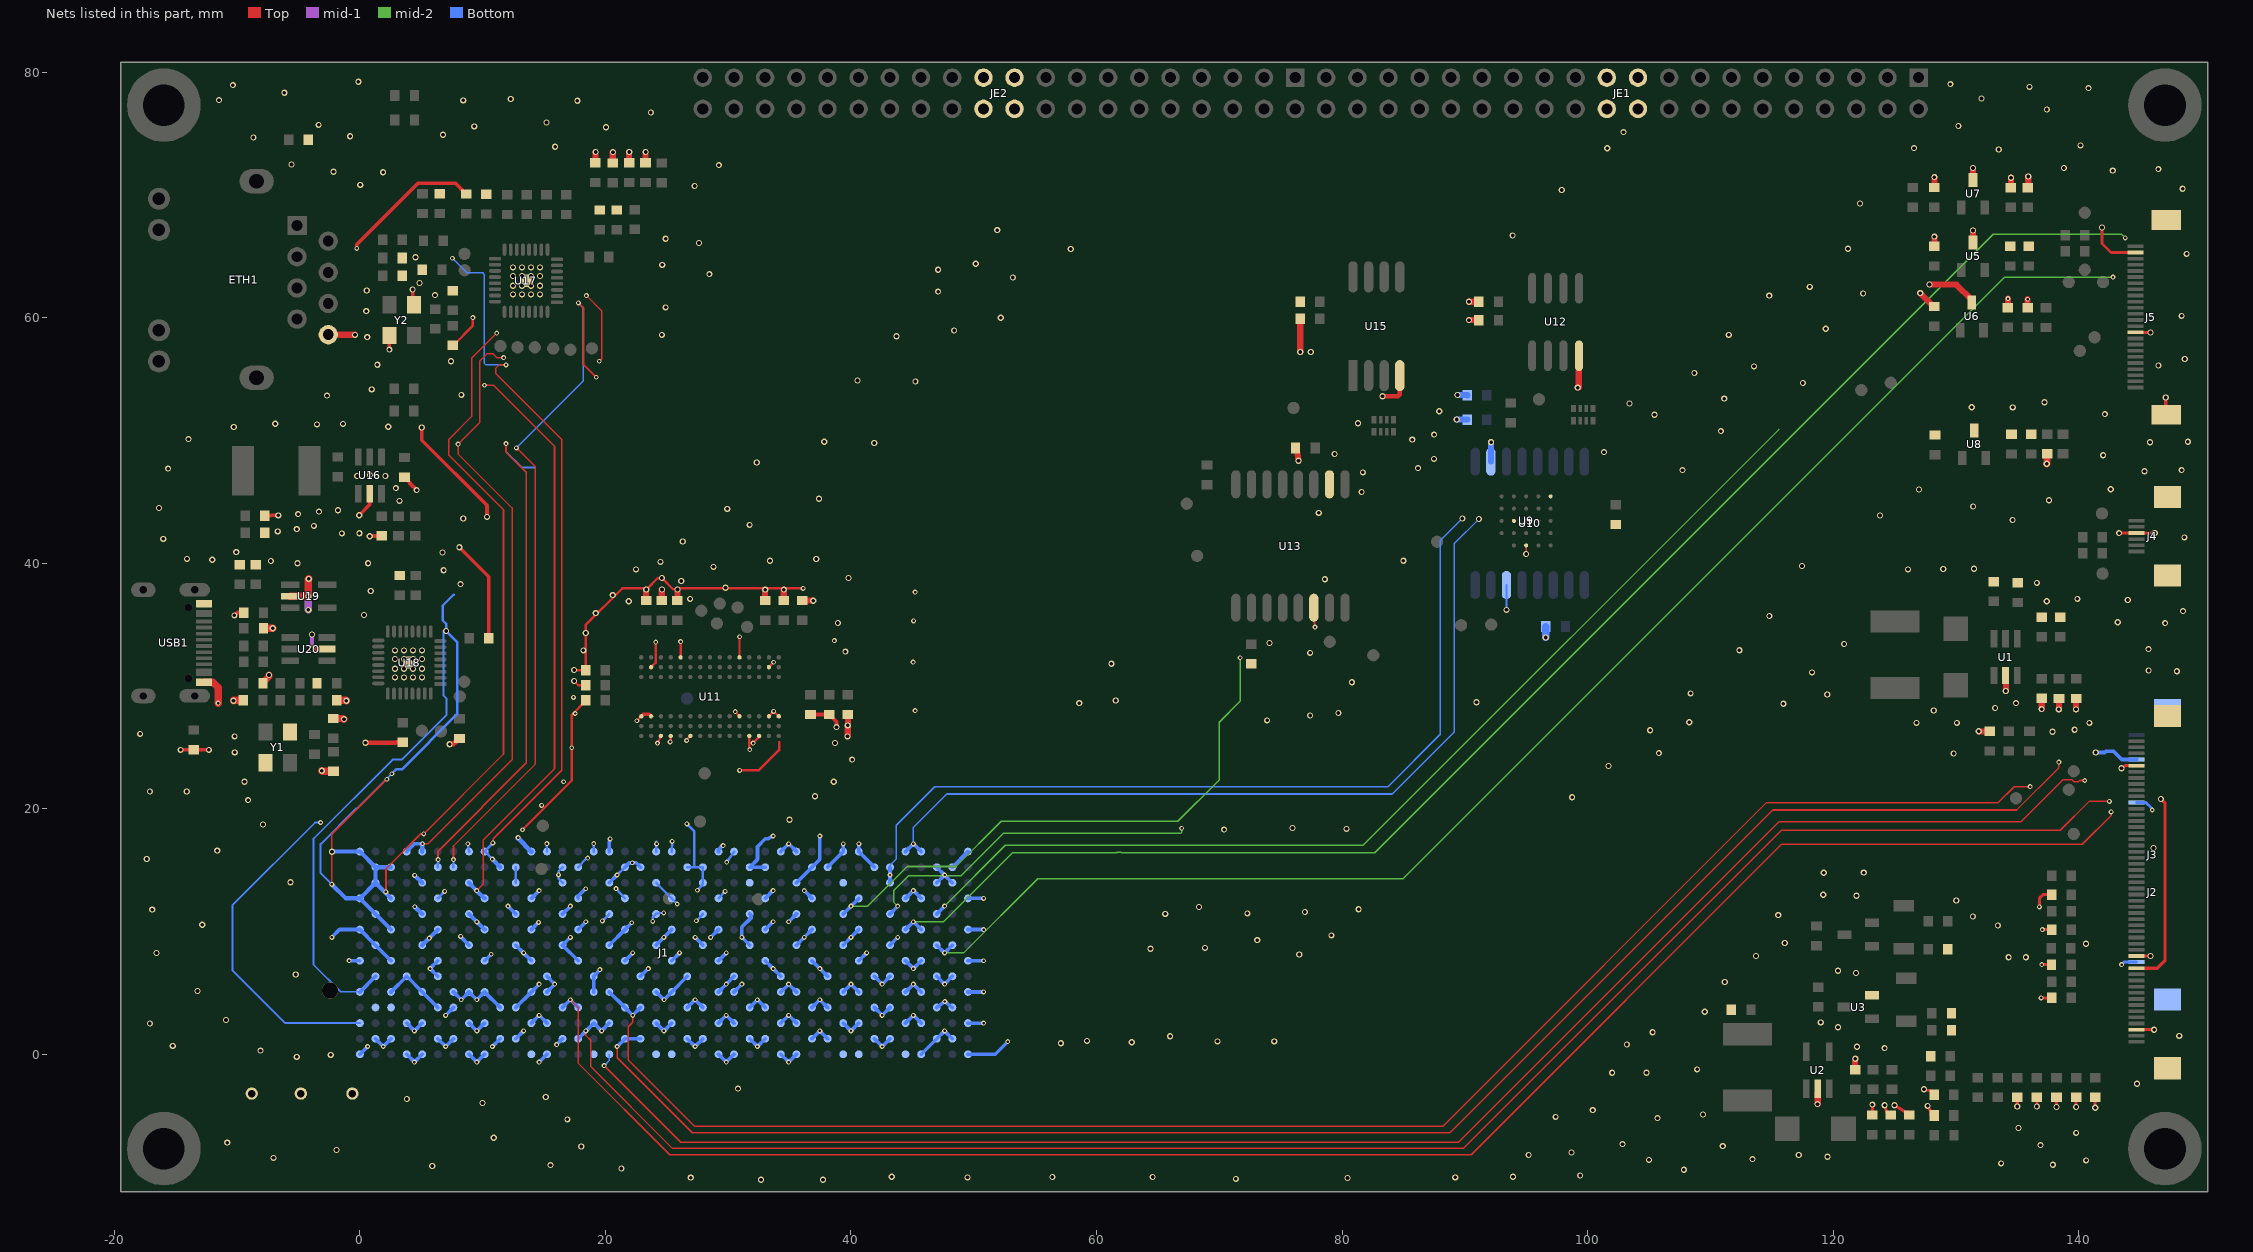
[diagram p0: the nets of this part, all layers, seen from the top]
# Altium PCB MISC105414.PcbDoc (part 6 of 11)
Units mm, origin at the board's own origin, x right, y up, seen from the top; angles counter-clockwise.
Board outline 170 x 92 mm, 6 copper layers (Top, GND, mid-1, mid-2, mid-3, Bottom), stack 1.231 mm thick; 238 components, 304 nets, 1456 pads, 1258 vias.
Unrouted connection lines stored in the file: 57.

## Via types
v1: diameter 0.4, hole 0.2, Top to Bottom, tented top, 618 vias
v2: diameter 0.5, hole 0.3, Top to Bottom, tented top, 522 vias
v3: diameter 0.5, hole 0.3, Top to Bottom, 41 vias
v4: diameter 1, hole 0.5, Top to Bottom, tented top, 36 vias
v5: diameter 0.7, hole 0.4, Top to Bottom, tented top, 34 vias
v6: diameter 1.3, hole 1.3, Top to Bottom, tented top, 3 vias
v7: diameter 4, hole 4, Top to Bottom, tented top, 2 vias
v8: diameter 3.3, hole 3.3, Top to Bottom, tented top, 2 vias

## Nets (pads, with @x,y where several pads share a name; then routed paths per layer and width w, separated by ;. In a path a pad name is that pad's centre, name@x,y a point inside that pad or via, vN(x,y) a via of type N, cw(c..) or ccw(c..) an arc to the next point about the centre after c; other vN are vias at no path point) (continued)
GND: C1.2 C3.2 C4.2 C5.1 C6.1 C7.1 C8.1 C9.2 C10.2 C11.2 C15.2 C17.2 C18.2 C19.1 C20.2 C21.2 C22.2 C27.2 C28.2 C29.2 C30.2 C31.2 C32.2 C33.2 C34.2 C35.1 C36.1 C37.1 C38.1 C39.2 C40.2 C41.2 C42.1 C43.1 C44.1 C45.2 C46.1 C47.1 C48.1 C49.1 C50.1 C51.1 C52.1 C53.1 C54.1 C55.1 C56.1 C65.2 C66.2 C67.1 C68.1 C69.2 C70.2 C71.2 C72.2 C73.1 C74.1 C75.1 C77.1 C78.1 C79.1 C80.2 C82.2 C83.2 C84.2 C85.2 C86.2 C87.1 C88.2 C89.1 C90.1 C91.1 C92.2 C93.2 C94.1 C95.1 ETH1.8 J1.A1 J1.A4 J1.A5 J1.A8 J1.A9 J1.A12 J1.A13 J1.A16 J1.A17 J1.A20 J1.A21 J1.A24 J1.A25 J1.A28 J1.A29 J1.A32 J1.A33 J1.A36 J1.A37 J1.A40 J1.B2 J1.B3 J1.B6 J1.B7 J1.B10 J1.B11 J1.B14 J1.B15 J1.B18 J1.B19 J1.B22 J1.B23 J1.B26 J1.B27 J1.B30 J1.B31 J1.B34 J1.B35 J1.B38 J1.B39 J1.C1 J1.C4 J1.C5 J1.C8 J1.C9 J1.C12 J1.C13 J1.C16 J1.C17 J1.C20 J1.C21 J1.C24 J1.C25 J1.C28 J1.C29 J1.C32 J1.C33 J1.C34 J1.C36 J1.C38 J1.C40 J1.D2 J1.D3 J1.D6 J1.D7 J1.D10 J1.D13 J1.D16 J1.D19 J1.D22 J1.D25 J1.D28 J1.D35 J1.D37 J1.D39 J1.E1 J1.E4 J1.E5 J1.E8 J1.E11 J1.E14 J1.E17 J1.E20 J1.E23 J1.E26 J1.E29 J1.E32 J1.E35 J1.E38 J1.E40 J1.F2 J1.F3 J1.F6 J1.F9 J1.F12 J1.F15 J1.F18 J1.F21 J1.F24 J1.F27 J1.F30 J1.F33 J1.F36 J1.F39 J1.G1 J1.G4 J1.G5 J1.G8 J1.G11 J1.G14 J1.G17 J1.G20 J1.G23 J1.G26 J1.G29 J1.G32 J1.G35 J1.G38 J1.G40 J1.H3 J1.H6 J1.H9 J1.H12 J1.H15 J1.H18 J1.H21 J1.H24 J1.H27 J1.H30 J1.H33 J1.H36 J1.H39 J1.J1 J1.J4 J1.J5 J1.J8 J1.J11 J1.J14 J1.J17 J1.J20 J1.J23 J1.J26 J1.J29 J1.J32 J1.J35 J1.J38 J1.J40 J1.K2 J1.K3 J1.K6 J1.K9 J1.K12 J1.K15 J1.K18 J1.K21 J1.K24 J1.K27 J1.K30 J1.K33 J1.K36 J1.K39 J1.L2 J1.L3 J1.L6 J1.L7 J1.L10 J1.L11 J1.L14 J1.L15 J1.L18 J1.L19 J1.L22 J1.L23 J1.L26 J1.L27 J1.L30 J1.L31 J1.L34 J1.L35 J1.L38 J1.L39 J1.M1 J1.M4 J1.M5 J1.M8 J1.M9 J1.M12 J1.M13 J1.M16 J1.M17 J1.M20 J1.M21 J1.M24 J1.M25 J1.M28 J1.M29 J1.M32 J1.M33 J1.M36 J1.M37 J1.M40 J1.Y1 J1.Y4 J1.Y5 J1.Y8 J1.Y9 J1.Y12 J1.Y13 J1.Y16 J1.Y17 J1.Y20 J1.Y21 J1.Y24 J1.Y25 J1.Y28 J1.Y29 J1.Y32 J1.Y33 J1.Y36 J1.Y37 J1.Y40 J1.Z2 J1.Z3 J1.Z6 J1.Z7 J1.Z10 J1.Z11 J1.Z14 J1.Z15 J1.Z18 J1.Z19 J1.Z22 J1.Z23 J1.Z26 J1.Z27 J1.Z30 J1.Z31 J1.Z34 J1.Z35 J1.Z38 J1.Z39 J2.0 J2.0/2 J2.5 J2.36 J2.38 J2.48 J3.0 J3.0/2 J3.3 J3.29 J3.36 J4.0 J4.0/2 J4.3 J5.0 J5.0/2 J5.2 J5.15 JE1.19 JE1.20 JE1.21 JE1.22 JE2.19 JE2.20 JE2.21 JE2.22 LR8.1 LR9.1 R2.1 R4.1 R5.1 R7.1 R9.1 R11.1 R12.1 R14.1 R16.1 R20.1 R22.1 R23.1 R31.2 R34.2 R37.2 R39.1 R46.1 R51.1 R54.1 TP1.1 TP2.1 TP3.1 U1.2 U2.2 U3.2 U5.3 U6.3 U7.3 U8.3 U9.B3 U9.C1 U9.E5 U10.6 U10.10 U11.A3 U11.B3 U11.B8 U11.C1 U11.D1 U11.E9 U11.F1 U11.L3 U11.L9 U11.M1 U11.N1 U11.P3 U11.P8 U11.R3 U12.4 U13.6 U13.10 U15.4 U16.2 U17.0 U18.0 U19.2 U20.2 USB1.1 USB1.12 Y1.2 Y1.4 Y2.2 Y2.4 | length 2103
  Top w0.127: v1(5.1,17.15) 5.55,17.15 12.4,24 12.4,44.5 8,48.9 v1(8,49.7) 9.75,51.45 9.75,56.45 10.35,57.05 10.854,57.05 11.154,56.75 v1(11.7,56.75) ; v1(5.2,17.95) 11.7,24.45 11.7,44.35 7.25,48.8 7.25,50.1 9.1,51.95 9.1,56.7 v1(11.15,58.75) ; v1(7.624,15.862) 7.624,16.974 14.3,23.65 14.3,47.85 v1(12.75,49.4) ; v1(9.504,13.329) 10.046,13.871 10.046,17.459 15.85,23.263 15.85,49.525 10.875,54.5 v1(10.15,54.5) ; v1(10.827,17.217) 10.871,17.26 10.871,17.566 16.45,23.145 16.45,50.075 11.05,55.475 11.05,55.864 11.336,56.15 v1(11.9,56.15) ; v1(17.145,4.445) 17.775,3.815 17.775,-0.716 25.241,-8.182 90.518,-8.182 115.8,17.1 140.3,17.1 142.65,19.45 v1(142.65,19.75) ; v1(18.415,1.905) 18.415,1.532 18.801,1.146 18.801,-1.002 25.47,-7.671 89.879,-7.671 115.8,18.25 138.5,18.25 140.85,20.6 v1(142.5,20.6) ; v1(18.45,61.8) 19.707,60.543 19.707,56.657 v1(19.5,56.45) ; v1(19.9,-0.925) 26.138,-7.163 89.479,-7.163 115.592,18.95 135.3,18.95 138.7,22.35 139.488,22.35 139.638,22.2 139.982,22.2 140.082,22.3 v1(140.5,22.3) ; v1(20.955,0.635) 20.955,-0.273 27.069,-6.387 88.801,-6.387 115.088,19.9 134.95,19.9 138.4,23.35 v1(138.4,23.8) ; v1(22.225,3.175) 22.225,2.615 21.861,2.252 21.861,-0.461 27.28,-5.879 88.199,-5.879 114.578,20.5 133.45,20.5 134.75,21.8 v1(136.05,21.8) ; U13.6@77.705,36.375 77.705,35.613 v1(77.8,34.8) ; U15.4@84.705,54.39 U15.4@84.705,55.279 ; v2(95,40.75) U9.C1@95,41.45
  Top w0.15: v1(-2.286,13.843) -2.286,17.914 v1(2.2,22.4) ; v1(2.125,13.225) 2.125,15.1 4.975,17.95 v1(5.2,17.95) ; v1(6.37,15.862) 6.37,16.55 13.55,23.73 13.55,47.4 11.9,49.05 v1(11.9,49.75) ; v1(17.8,61.2) 18.225,60.775 18.225,56.175 v1(19.25,55.15)
  Top w0.2: v2(7.314,25.251) 7.362,25.27 7.785,25.439 8.117,25.439 C70.2@8.117,25.72 ; C85.2@7.55,57.75 7.601,57.75 9.2,59.349 v1(9.2,60) ; v1(13.245,18.29) 17.258,22.304 v1(17.258,24.972) 17.258,27.639 18.393,28.774 C51.1@18.393,28.825 ; v3(17.45,30.4) 17.79,30.06 C48.1@18.393,30.06 ; v3(17.45,31.3) 17.455,31.295 C50.1@18.393,31.295 18.393,32.9 18.393,34.965 21.374,37.946 23.423,37.946 24.25,38.773 24.573,38.773 v2(24.6,38.8) 25.526,37.874 25.791,37.874 25.863,37.946 29.775,37.946 v1(36.11,37.946) ; v1(22.558,27.166) U11.A3@22.92,27.533 ; U11.B8@23.72,31.533 24.098,31.911 24.098,33.537 24.079,33.556 24.051,33.583 24.094,33.583 v1(24.101,33.577) ; v1(24.243,25.344) U11.C1@24.52,25.933 ; v1(25.268,25.441) 25.32,25.441 U11.D1@25.32,25.933 ; U11.E9@26.12,32.333 26.12,33.602 v1(26.127,33.608) ; v1(26.62,25.561) 26.607,25.561 26.607,25.612 26.612,25.617 26.612,25.624 U11.F1@26.92,25.933 ; v1(30.576,27.909) U11.L3@30.92,27.533 ; U11.L9@30.92,32.333 30.92,34.008 v1(30.924,34.008) ; v1(30.93,23.119) 32.483,23.119 34.143,24.779 34.143,25.436 ; U11.M1@31.72,25.933 31.72,24.86 v1(31.758,24.822) ; v1(32.027,25.347) 32.52,25.841 U11.N1@32.52,25.933 ; U11.P3@33.32,27.533 v1(33.706,27.931) U11.R3@34.12,27.533 ; U11.P8@33.32,31.533 v1(33.706,31.936)
  Top w0.25: C17.2@123.2,-4.95 v2(123.2,-4.1) ; v2(124.2,-4.15) 124.484,-4.95 C18.2@124.7,-4.95 ; v2(125,-4.15) 125.893,-4.694 126.2,-4.694 C19.1@126.2,-4.95 ; v2(127.4,-2.85) 128.238,-3.039 C22.2@128.238,-3.288 ; v2(127.7,-4.2) 127.982,-4.681 127.982,-4.988 R22.1@128.238,-4.988 ; v2(135,-4.25) C3.2@135,-3.5 ; v2(136.6,-4.25) C4.2@136.6,-3.5 ; v1(136.8,12) 136.8,12.7 137.1,13 R4.1@137.8,13 ; v1(136.95,4.6) R11.1@137.8,4.6 ; v1(137,7.3) R9.1@137.792,7.3 ; v1(137.05,10.15) R2.1@137.8,10.15 ; v2(138.2,-4.3) C5.1@138.2,-3.5 ; v2(139.8,-4.3) C6.1@139.8,-3.5 ; v2(141.35,-4.35) R16.1@141.35,-3.5 ; v2(141.9,67.35) 141.9,66.05 142.64,65.31 J5.2@144.63,65.31 ; v2(143.3,42.45) 143.3,42.46 J4.3@144.733,42.46 146.2,42.46 v2(146.2,42.45) ; v2(143.5,23.3) 143.568,23.3 143.778,23.51 J2.5@144.73,23.51 ; J5.15@144.63,58.81 145.85,58.81 v2(145.85,58.8) ; J2.48@144.73,2.01 146.15,2.01 v2(146.15,2) ; J2.38@144.73,7.01 146.412,7.01 147.05,7.648 147.05,20.45 v2(146.7,20.8) ; J2.36@144.73,8.01 145.85,8.01 v2(145.85,8) ; v2(147.1,53.5) 147.1,52.106 J5.0/2@147.127,52.106
  Top w0.3: v3(-14.6,24.8) -14.588,24.812 LR8.1@-13.53,24.812 -12.312,24.812 v3(-12.3,24.8) ; v2(-10.225,35.75) -10.191,35.75 -9.96,35.98 R46.1@-9.455,35.98 ; C84.2@-7.745,43.857 -7.264,43.857 -7.221,43.9 v2(-6.65,43.9) ; v3(-3.9,33) -3.89,33.01 U20.2@-2.67,33.01 ; v1(-0.255,65.645) -0.255,65.958 4.75,70.963 7.761,70.963 R39.1@8.652,70.073 ; v2(-0.053,43.91) 0.812,44.775 U16.2@0.812,45.661 ; v3(0.8,42.2) 0.825,42.225 R31.2@1.771,42.225 ; v3(2.4,57.4) Y2.4@2.4,58.55 ; C69.2@3.637,47.016 4.088,46.564 4.088,46.492 v2(4.625,45.955) ; v3(4.3,62.3) 4.3,61.15 Y2.2@4.4,61.05 ; v2(5.043,51.053) 5.043,50.026 10.354,44.715 v2(10.354,43.774) ; v3(8.1,41.3) 10.498,38.902 C77.1@10.498,33.893 ; U11.A3@22.92,27.533 22.935,27.533 23.089,27.686 23.567,27.686 U11.B3@23.72,27.533 ; C49.1@36.708,27.679 C46.1@38.228,27.679 38.825,27.082 v3(38.825,26.65)
  Top w0.4: v3(0.45,25.375) 2.917,25.375 2.961,25.419 C80.2@3.492,25.419 ; v2(7.314,25.251) 7.333,25.27 7.362,25.27 7.616,25.27 7.785,25.439 8.066,25.72 C70.2@8.117,25.72 ; v2(83.3,53.6) 84.555,53.6 84.705,53.75 U15.4@84.705,54.39
  Top w0.5: ETH1.8@-2.575,58.615 -0.415,58.615 v3(-0.4,58.6) ; C90.1@19.187,72.613 19.187,73.487 v3(19.2,73.5) ; C74.1@20.6,72.6 v3@20.6,73.474 ; C71.2@21.934,72.614 v3@21.934,73.488 ; C78.1@23.267,72.614 v3@23.267,73.488 ; C45.2@23.317,36.965 v3@23.317,37.839 ; C53.1@24.59,36.965 v3@24.59,37.839 ; C52.1@25.863,36.965 v3@25.863,37.839 ; C55.1@33.006,36.959 v3@33.006,37.834 ; C54.1@34.526,36.959 v3@34.526,37.834 ; C47.1@36.046,36.959 v3@36.92,36.959 ; v2(39.725,25.9) 39.735,25.91 v3(39.735,26.792) 39.748,26.805 C56.1@39.748,27.679 ; C67.1@76.213,49.387 76.344,49.387 76.344,49.205 v2(76.45,48.35) ; v2(76.6,57.2) 76.6,58.459 C66.2@76.6,59.9 ; v2(90.35,59.8) C40.2@91.15,59.8 ; v2(90.35,61.3) C43.1@91.15,61.3 ; v2(99.2,54.3) 99.281,54.3 99.281,56.9 U12.4@99.305,56.9 ; v3@118.75,-4.049 U2.2@118.75,-3.175 ; R20.1@121.8,-1.25 v3@121.8,-0.376 ; v2(127.1,62) 128.196,60.908 C28.2@128.246,60.908 ; v2(127.85,62.7) 130.05,62.7 131.3,61.45 U6.3@131.3,61.225 ; C27.2@128.246,65.808 128.25,65.808 v2(128.25,66.6) ; C29.2@128.246,70.608 128.25,70.608 v2(128.25,71.45) ; U5.3@131.4,66.125 v2(131.4,67.1) ; U7.3@131.4,71.225 v2(131.4,72.2) ; v3@131.876,26.3 R7.1@132.75,26.3 ; v3@134.075,29.601 U1.2@134.075,30.475 ; C32.2@134.243,60.817 134.25,60.817 v1(134.25,61.55) ; C33.2@134.47,70.59 134.5,70.59 v2(134.5,71.4) ; C36.1@135.846,60.808 135.85,60.808 v1(135.85,61.5) ; C37.1@135.87,70.59 135.9,70.59 v2(135.9,71.5) ; v3@137,28.126 C7.1@137,29 ; v3@138.4,28.108 R14.1@138.4,28.982 ; v3@139.8,28.108 R12.1@139.8,28.982
  Top w0.6: USB1.12@-12.707,30.31 -11.985,30.31 -11.55,29.875 v1(-11.55,28.6) ; v3(-10.3,28.8) -10.264,28.836 R34.2@-9.491,28.836 ; R54.1@-7.892,30.236 -7.892,30.286 -7.4,30.778 v3(-7.4,30.9) ; R51.1@-7.855,34.705 -7.105,34.705 v3(-7.1,34.7) ; U19.2@-5.658,37.317 -4.217,37.317 v3(-4.2,37.3) -4.2,38.688 v3(-4.161,38.727) ; v3(-3.1,23.1) -3.05,23.05 C82.2@-2.15,23.05 ; C83.2@-2.174,27.35 -1.377,27.35 -1.327,27.3 v2(-1.3,27.3) ; R37.2@-1.892,28.836 -1.163,28.836 -1.127,28.8 v2(-1.1,28.8) ; v2(137.4,48.1) 137.43,48.13 R23.1@137.43,48.91
  mid-1 w0.3: v3(-3.9,33) v3(-3.9,34.2)
  mid-1 w0.6: v3(-4.2,36.2) v3(-4.2,37.3)
  mid-2 w0.127: v1(40.005,12.065) 41.357,12.065 44.587,15.295 48.564,15.295 52.243,18.974 66.624,18.974 70,22.35 70,27.05 71.7,28.75 v1(71.7,32.3) ; v1(43.815,12.065) 43.474,12.406 43.474,13.32 44.689,14.534 48.958,14.534 52.424,18 66.855,18 66.929,18.075 v1(66.929,18.415) ; v1(45.085,10.795) 47.542,10.795 53.165,16.418 61.641,16.418 61.698,16.475 62,16.475 62.057,16.418 82.658,16.418 133.04,66.8 143.5,66.8 v1(143.8,66.5) ; v1(47.625,8.255) 49.165,8.255 55.209,14.299 84.966,14.299 133.967,63.3 v1(142.8,63.3) ; v1(47.625,12.065) 52.578,17.018 81.714,17.018 115.589,50.893
  Bottom w0.127: v1(7.542,64.845) 8.731,63.656 10,63.656 10.118,63.538 10.118,56.3 10.268,56.15 v1(11.9,56.15) ; v1(12.75,49.4) 18.2,54.85 18.2,60.8 v1(17.8,61.2) ; v1(19.9,-0.925) 20.32,-0.505 J1.Y24@20.32,0 ; J1.L6@43.18,15.24 43.18,15.405 43.688,15.913 43.688,18.663 46.825,21.8 83.741,21.8 88,26.059 88,41.85 v2(89.8,43.65) ; v1(45.085,17.145) 45.085,18.485 47.8,21.2 84.1,21.2 89.15,26.25 89.15,41.6 v2(91.15,43.6) ; U10.6@93.395,38.225 93.397,38.225 93.397,36.2 v2(93.4,36.2)
  Bottom w0.15: v1(-3.197,18.882) -3.648,18.882 -10.383,12.147 -10.383,6.827 -6.096,2.54 J1.A40@0,2.54 ; v1(-2.286,13.843) -3.202,14.759 -3.202,17.123 -0.3,20.025 -0.225,20.025 v1(2.6,22.85) ; J1.C40@0,5.08 -0.437,5.091 -0.8,5.1 -1.568,5.1 -3.777,7.309 -3.777,17.564 2.666,24.008 3.403,24.008 7.066,27.671 7.066,28.975 6.802,29.239 v3@6.802,34.478 ; v1(11.9,49.75) 11.9,49.07 13.17,47.8 14.25,47.8
  Bottom w0.2: v1(2.6,22.85) 2.953,23.203 3.416,23.203 7.923,27.71 7.923,33.583 v3(7.028,34.478) 7.028,35.065 6.75,35.343 6.75,36.55 7.65,37.45 ; J1.J35@6.35,12.7 v1(6.908,13.276) ; J1.L35@6.35,15.24 v1(6.37,15.862) ; J1.L34@7.62,15.24 v1(7.624,15.862) ; v1(8.8,17.15) J1.M33@8.89,16.51 ; v1(10.797,15.891) 10.178,16.51 J1.M32@10.16,16.51 v1(10.827,17.217) ; J1.K30@12.7,13.97 J1.L30@12.7,15.24 ; v1(15.236,17.168) J1.M28@15.24,16.51 ; J1.K27@16.51,13.97 16.51,13.974 16.177,14.307 v1(16.177,14.612) 16.187,14.622 16.187,14.912 16.51,15.236 J1.L27@16.51,15.24 ; J1.L26@17.78,15.24 18.444,15.966 v1(18.559,15.98) ; J1.M25@19.05,16.51 v1(19.051,17.153) ; v1(19.747,10.865) J1.H24@20.32,11.43 ; v1(20.861,13.498) J1.J23@21.59,12.7 ; v1(20.955,14.605) J1.L23@21.59,15.24 ; v1(23.859,10.827) 23.859,11.159 J1.H21@24.13,11.43 v1(24.752,11.523) ; J1.K21@24.13,13.97 J1.J20@25.4,12.7 v1(25.848,12.243) ; J1.M21@24.13,16.51 24.13,17.303 24.151,17.324 v1(24.169,17.133) ; J1.M20@25.4,16.51 v1(25.427,17.34) ; v1(26.64,18.77) 27.223,18.187 27.223,15.24 ; J1.L19@26.67,15.24 27.223,15.24 ; v1(27.412,10.874) J1.H18@27.94,11.43 ; v1(27.497,13.362) 27.545,13.375 27.927,13.836 J1.K18@27.94,13.97 J1.L18@27.94,15.24 27.223,15.24 ; J1.J17@29.21,12.7 v1(29.743,13.267) ; v1(29.883,15.646) J1.M16@30.48,16.51
  Bottom w0.25: v1(143.5,7.3) 143.71,7.51 J3.3@144.73,7.51 ; J3.29@144.73,20.51 145.48,20.51 145.971,20.019 145.971,19.929 v1(146,19.9)
  Bottom w0.3: v1(-2.286,9.525) -1.651,10.16 J1.G40@0,10.16 J1.F39@1.27,8.89 J1.E38@2.54,7.62 ; v1(-0.875,7.632) J1.E40@0,7.62 ; J1.Y40@0,0 v1(0.635,0.635) ; J1.C40@0,5.08 J1.D39@1.27,6.35 ; J1.J40@0,12.7 J1.H39@1.27,11.43 J1.G38@2.54,10.16 ; J1.Z39@1.27,1.27 v1(1.905,0.635) J1.Z38@2.54,1.27 ; J1.C38@2.54,5.08 J1.D37@3.81,6.35 J1.C36@5.08,5.08 J1.B35@6.35,3.81 ; J1.Y37@3.81,0 v1(4.445,-0.635) J1.Y36@5.08,0 ; J1.A37@3.81,2.54 v1(4.445,1.905) J1.A36@5.08,2.54 ; J1.M37@3.81,16.51 4.45,17.15 v1(5.1,17.15) ; J1.Z35@6.35,1.27 v1(6.985,0.635) J1.Z34@7.62,1.27 ; J1.D35@6.35,6.35 v1(5.715,6.985) J1.E35@6.35,7.62 ; v1(6.985,3.175) J1.B34@7.62,3.81 ; J1.C34@7.62,5.08 v1(8.255,4.445) J1.C33@8.89,5.08 v1(9.525,4.445) J1.C32@10.16,5.08 J1.B31@11.43,3.81 ; v1(8.2,9.6) J1.F33@8.89,8.89 ; J1.Y33@8.89,0 v1(9.525,-0.635) J1.Y32@10.16,0 ; J1.A33@8.89,2.54 v1(9.525,1.905) J1.A32@10.16,2.54 ; J1.E32@10.16,7.62 v1(10.7,8.15) ; v1(10.795,0.635) J1.Z31@11.43,1.27 ; J1.Z30@12.7,1.27 v1(13.335,1.905) ; J1.B30@12.7,3.81 J1.C29@13.97,5.08 v1(14.605,5.715) ; J1.F30@12.7,8.89 v1(13.335,8.255) J1.E29@13.97,7.62 ; J1.A29@13.97,2.54 v1(14.605,3.175) J1.A28@15.24,2.54 ; J1.G29@13.97,10.16 v1(14.55,10.75) ; v1(14.605,-0.635) J1.Y28@15.24,0 ; J1.C28@15.24,5.08 v1(15.875,5.715) J1.D28@15.24,6.35 ; v1(16.032,0.792) J1.Z27@16.51,1.27 ; J1.B27@16.51,3.81 v1(17.145,4.445) J1.B26@17.78,3.81 ; v1(17.145,9.525) J1.F27@16.51,8.89 J1.E26@17.78,7.62 ; J1.Z26@17.78,1.27 v1(18.415,1.905) J1.A25@19.05,2.54 v1(19.685,1.905) J1.A24@20.32,2.54 ; J1.C25@19.05,5.08 J1.D25@19.05,6.35 v1(19.553,6.894) ; J1.C24@20.32,5.08 J1.B23@21.59,3.81 v1(22.225,3.175) J1.B22@22.86,3.81 ; J1.F24@20.32,8.89 J1.G23@21.59,10.16 v1(22.146,10.716) ; v1(20.955,0.635) J1.Z23@21.59,1.27 J1.Z22@22.86,1.27 ; J1.E23@21.59,7.62 v1(22.225,8.255) ; J1.L23@21.59,15.24 21.929,15.579 22.174,15.579 v1(22.193,15.598) 22.502,15.598 J1.L22@22.86,15.24 ; J1.D22@22.86,6.35 v1(23.495,6.985) ; J1.A21@24.13,2.54 v1(24.765,1.905) J1.A20@25.4,2.54 ; J1.C21@24.13,5.08 v1(24.775,4.444) J1.C20@25.4,5.08 J1.D19@26.67,6.35 ; J1.F21@24.13,8.89 v1(24.765,9.525) J1.G20@25.4,10.16 ; J1.E20@25.4,7.62 v1(26.035,8.255) ; J1.Z19@26.67,1.27 v1(27.305,0.635) J1.Z18@27.94,1.27 ; J1.B19@26.67,3.81 v1(27.305,4.445) J1.B18@27.94,3.81 ; v1(27.305,9.525) J1.F18@27.94,8.89 ; v1(28.575,9.525) J1.G17@29.21,10.16 ; J1.Y17@29.21,0 v1(29.845,-0.635) J1.Y16@30.48,0 ; J1.A17@29.21,2.54 v1(29.845,3.175) J1.A16@30.48,2.54 ; J1.C17@29.21,5.08 v1(29.845,5.715) J1.D16@30.48,6.35 ; J1.E17@29.21,7.62 v1(29.845,8.255) ; J1.C16@30.48,5.08 v1(31.115,5.715) ; J1.Z15@31.75,1.27 v1(32.385,0.635) J1.Z14@33.02,1.27 ; J1.B15@31.75,3.81 v1(32.385,4.445) J1.B14@33.02,3.81 ; J1.F15@31.75,8.89 v1(31.115,9.525) 31.115,10.359 31.854,11.098 31.854,11.326 J1.H15@31.75,11.43 ; J1.E14@33.02,7.62 v1(33.655,6.985) J1.D13@34.29,6.35 ; J1.G14@33.02,10.16 v1(33.655,10.795) ; J1.J14@33.02,12.7 v1(33.655,13.335) ; J1.L14@33.02,15.24 J1.L15@31.75,15.24 32.385,15.875 32.385,16.91 33.022,17.547 33.251,17.547 v1(33.655,17.78) ; J1.Y13@34.29,0 v1(34.925,-0.635) J1.Y12@35.56,0 ; J1.A13@34.29,2.54 v1(34.925,3.175) J1.A12@35.56,2.54 ; J1.C13@34.29,5.08 v1(34.925,5.715) J1.C12@35.56,5.08 ; J1.M13@34.29,16.51 v1(34.925,17.145) J1.M12@35.56,16.51 ; v1(34.925,10.795) J1.H12@35.56,11.43 ; J1.F12@35.56,8.89 v1(36.195,9.525) J1.G11@36.83,10.16 ; J1.K12@35.56,13.97 J1.L11@36.83,15.24 37.465,15.875 v1(37.465,17.78) ; v1(36.195,13.335) J1.J11@36.83,12.7 ; J1.Z11@36.83,1.27 v1(37.465,1.905) J1.Z10@38.1,1.27 ; J1.B11@36.83,3.81 v1(37.465,4.445) J1.B10@38.1,3.81 ; J1.E11@36.83,7.62 v1(37.465,6.985) J1.D10@38.1,6.35 ; J1.L10@38.1,15.24 J1.M9@39.37,16.51 v1(39.37,17.145) ; J1.A9@39.37,2.54 v1(40.005,1.905) J1.A8@40.64,2.54 ; J1.C9@39.37,5.08 v1(40.005,5.715) J1.C8@40.64,5.08 ; J1.F9@39.37,8.89 v1(40.005,9.525) J1.G8@40.64,10.16 ; J1.H9@39.37,11.43 v1(40.005,12.065) J1.J8@40.64,12.7 ; J1.E8@40.64,7.62 v1(41.275,8.255) ; v1(40.64,17.145) J1.M8@40.64,16.51 J1.L7@41.91,15.24 ; J1.Z7@41.91,1.27 v1(42.545,0.635) J1.Z6@43.18,1.27 ; J1.B7@41.91,3.81 v1(42.545,3.175) J1.B6@43.18,3.81 ; J1.D7@41.91,6.35 v1(42.545,5.715) J1.D6@43.18,6.35 ; J1.F6@43.18,8.89 v1(43.815,9.525) ; J1.H6@43.18,11.43 v1(43.815,12.065) ; J1.K6@43.18,13.97 v1(43.18,14.605) J1.L6@43.18,15.24 ; J1.A5@44.45,2.54 v1(45.085,3.175) J1.A4@45.72,2.54 ; J1.C5@44.45,5.08 v1(45.085,5.715) J1.C4@45.72,5.08 ; J1.E5@44.45,7.62 v1(45.085,6.985) J1.E4@45.72,7.62 ; J1.G5@44.45,10.16 v1(45.085,10.795) J1.G4@45.72,10.16 ; J1.J5@44.45,12.7 v1(45.085,13.335) J1.J4@45.72,12.7 ; J1.M5@44.45,16.51 v1(45.085,17.145) J1.M4@45.72,16.51 ; J1.Y4@45.72,0 J1.Z3@46.99,1.27 v1(47.625,1.905) J1.Z2@48.26,1.27 ; J1.B3@46.99,3.81 v1(47.65,4.3) J1.B2@48.26,3.81 ; J1.D3@46.99,6.35 v1(47.625,5.715) J1.D2@48.26,6.35 ; J1.F3@46.99,8.89 v1(47.625,8.255) J1.F2@48.26,8.89 ; J1.H3@46.99,11.43 v1(47.625,12.065) ; J1.K3@46.99,13.97 v1(47.625,14.605) ; J1.L3@46.99,15.24 v1(47.625,14.605) ; J1.K2@48.26,13.97 v1(47.625,14.605) ; J1.L2@48.26,15.24 J1.M1@49.53,16.51 ; J1.Y1@49.53,0 51.75,0 v1(52.775,1.025) ; J1.A1@49.53,2.54 v1(50.8,2.54) ; J1.C1@49.53,5.08 v1(50.8,5.08) ; J1.E1@49.53,7.62 v1(50.8,7.62) ; J1.G1@49.53,10.16 v1(50.8,10.16) ; J1.J1@49.53,12.7 v1(50.8,12.7) ; v3(141.4,24.575) 142.102,24.575 142.202,24.675 142.85,24.675 143.515,24.01 J3.36@144.73,24.01
  Bottom w0.305: v1(12.065,12.065) J1.H30@12.7,11.43 ; J1.J29@13.97,12.7 v1(14.605,13.335) ; J1.H27@16.51,11.43 v1(17.145,12.065) ; J1.G26@17.78,10.16 v1(18.415,10.795) ; J1.J26@17.78,12.7 17.764,12.872 18.375,13.484 v1(18.401,13.481) ; J1.K24@20.32,13.97 v1(20.955,14.605) ; J1.M24@20.32,16.51 20.32,17.333 20.333,17.333 ; v1(20.383,17.553) 20.333,17.333 ; J1.M17@29.21,16.51 29.21,16.663 29.548,17.001 v1(29.591,17.001) ; 20.333,17.333 20.334,17.327 20.331,17.324 20.333,17.333
  Bottom w0.35: v1(-2.286,13.843) -1.143,12.7 J1.J40@0,12.7 J1.K39@1.27,13.97 ; v3(-2.275,16.5) -2.265,16.51 J1.M40@0,16.51 J1.L39@1.27,15.24 ; J1.J38@2.54,12.7 J1.K39@1.27,13.97 ; J1.L38@2.54,15.24 J1.L39@1.27,15.24 ; v1(4.457,14.576) 4.761,14.271 4.779,14.271 J1.K36@5.08,13.97 ; v1(4.471,12.021) J1.H36@5.08,11.43 ; J1.F36@5.08,8.89 J1.G35@6.35,10.16 ; J1.H33@8.89,11.43 J1.G32@10.16,10.16 ; J1.K33@8.89,13.97 v1(9.504,13.329) J1.J32@10.16,12.7 ; v1(10.797,15.891) 11.129,15.559 11.129,15.541 J1.L31@11.43,15.24 ; J1.K39@1.27,13.97 J1.L39@1.27,15.24
  Bottom w0.4: J1.M36@5.08,16.51 5.08,17.13 v1(5.1,17.15) ; v1(12.891,17.657) 12.891,17.589 J1.M29@13.97,16.51
  Bottom w0.5: v2(89.35,51.7) C42.1@90.2,51.7 ; v2(89.4,53.7) 90.2,53.7 C44.1@90.2,53.675 ; U10.10@92.125,48.275 92.125,49.037 v2(92.15,49.85)
  Bottom w0.6: v2(96.6,33.95) 96.6,34.799 C41.2@96.6,34.85
  other v1: 5.654,9.456 9.532,10.789 14.8,20.275 16.6,22.2 17.532,27.758 45.234,27.997 17.4,29.075 45.059,31.947 38.65,33.7 45.102,35.308 45.234,37.647
  other v2: 32.675,-10.225 37.725,-10.225 71.35,-10.15 80.45,-10.075 26.95,-10.05 49.5,-10.025 89.225,-10.025 56.403,-9.994 64.575,-10 43.325,-9.975 93.925,-9.975 99.4,-9.875 107.849,-9.409 21.3,-9.3 5.9,-9.1 15.527,-9.029 137.9,-9 133.692,-8.885 140.615,-8.638 105,-8.6 113.442,-8.54 -7.042,-8.434 119.545,-8.341 95.2,-8.2 117.2,-8.2 98.7,-8 -1.9,-7.8 18.03,-7.508 111.019,-7.482 136.9,-7.4 102.853,-7.315 -10.8,-7.2 10.9,-6.8 139.8,-6.4 135.1,-6 16.9,-5.3 105.7,-5.2 97.4,-5.1 109.4,-4.9 100.422,-4.547 9.981,-3.974 3.825,-3.641 15.134,-3.483 30.8,-2.8 144.754,-2.4 102,-1.5 104.8,-1.5 108.926,-1.225 -5.142,-0.212 -2.373,-0.047 -8.1,0.3 124.2,0.5 121.942,0.613 -15.246,0.689 103.2,0.8 57.1,0.9 62.873,0.981 69.857,1.051 74.486,1.054 59.235,1.096 65.999,1.466 148.2,1.5 105.3,1.8 120.4,2.2 -17.111,2.504 119,2.6 -10.9,2.8 109.543,3.468 -13.234,5.155 111.173,5.892 -5.221,6.498 121.867,6.622 120.4,6.8 134.3,7.9 135.7,7.9 113.729,8.007 76.52,8.13 -16.571,8.247 64.4,8.6 68.841,8.672 140.6,9 116.068,9.062 73.1,9.3 79.133,9.688 133.426,10.496 -12.841,10.554 131.386,11.223 115.535,11.334 65.6,11.437 72.291,11.479 76.976,11.588 -16.915,11.781 81.357,11.818 68.345,12 130.033,12.526 121.909,12.915 119.2,13 -5.653,14.013 119.237,14.793 122.5,14.8 -17.356,15.903 -11.614,16.59 146.1,16.8 70.4,18.3 80.361,18.364 75.966,18.426 -7.889,18.717 35,19.1 -9.1,20.7 98.746,20.935 37.075,21.024 -17.111,21.4 -14.1,21.4 -9.4,22.2 38.6,22.2 101.7,23.489 40.1,24 105.811,24.527 129.823,24.506 -10.191,24.59 38.704,25.36 -10.2,25.9 -17.9,26.1 137.875,26.275 105.1,26.4 139.679,26.431 126.8,27 130.081,26.994 140.875,27 108.286,27.042 73.9,27.2 77.4,27.6 79.7,27.8 128.2,28 133.2,28.2 115.949,28.557 58.6,28.6 134.9,28.6 90.961,28.68 61.571,28.815 119.531,29.31 108.4,29.4 80.8,30.3 2.867,30.7 3.6,30.7 4.333,30.7 5.067,30.7 118.287,31.111 148,31.2 145.704,31.263 2.867,31.4 3.6,31.4 4.333,31.4 5.067,31.4 61.21,31.808 2.867,32.2 3.6,32.2 4.333,32.2 5.067,32.2 77.4,32.7 39.544,32.796 2.867,32.9 3.6,32.9 4.333,32.9 5.067,32.9 18.2,32.9 112.368,32.912 145.7,33 120.903,33.427 74.1,33.5 18.395,34.319 147.05,35.12 38.933,35.132 143.193,35.193 114.813,35.7 0.341,35.778 19.211,35.936 148.5,36.1 21.9,36.9 137.4,36.9 144,37 26.9,37.1 139.9,37.1 20.6,37.4 0.889,37.742 29.775,38 8.2,38.3 136.6,38.4 26.175,38.549 78.6,38.7 39.8,38.8 6.825,39.425 22.489,39.501 126.1,39.5 128.971,39.534 131.48,39.551 28.8,39.7 117.472,39.774 -5.075,40 0.675,40 24.486,40.109 -7.25,40.175 33.4,40.2 85,40.2 -12.027,40.283 37.175,40.35 -14.086,40.356 6.733,40.87 -10.075,40.9 26.3,41.775 -16.016,41.985 148.615,42.107 -1.465,42.434 -0.043,42.443 -6.686,42.597 -5.138,42.779 -3.752,43.045 31.75,43.125 134.623,43.515 8.417,43.648 123.819,43.891 -5.028,43.999 78.1,44.1 -3.325,44.2 -1.784,44.311 29.925,44.425 -16.361,44.496 131.41,44.62 3.22,45.079 137.585,45.135 37.395,45.248 81.6,45.8 127,46 142.619,46.029 2.931,46.118 -0.225,47.1 2.075,47.1 0.824,47.177 81.7,47.4 145.37,47.497 107.734,47.583 148.391,47.582 -15.618,47.706 86.195,47.747 32.325,48.2 87.5,48.5 142,48.8 79.4,48.9 101.336,49.047 41.9,49.8 145.82,49.853 37.821,49.89 148.9,49.9 85.718,50.068 -13.965,50.111 87.501,50.478 110.862,50.76 -10.275,51.1 2.31,51.119 -3.496,51.313 -1.375,51.35 -6.891,51.367 81.3,51.4 105.455,52.095 142.142,52.14 87.925,52.383 134.633,52.696 131.3,52.7 103.41,53.014 137.225,53.107 111.136,53.406 -2.678,53.652 8.268,53.716 0.968,54.161 117.536,54.676 45.25,54.8 40.528,54.891 108.7,55.5 113.556,56.036 146.5,56.1 1.421,56.168 7.425,56.45 148.65,56.629 77.45,57.2 0.601,58.415 43.716,58.488 24.6,58.6 111.5,58.6 48.404,58.951 119.4,59.1 52.2,60 148.393,60.145 0.516,60.535 24.908,60.841 114.8,61.8 6.125,61.836 12.467,61.9 13.2,61.9 13.933,61.9 14.667,61.9 122.448,61.975 47.1,62.125 0.559,62.217 118.104,62.513 12.467,62.6 13.2,62.6 13.933,62.6 14.667,62.6 4.85,62.825 53.191,63.274 12.467,63.4 13.2,63.4 13.933,63.4 14.667,63.4 28.463,63.549 47.1,63.9 12.467,64.1 13.2,64.1 13.933,64.1 14.667,64.1 24.625,64.3 50.161,64.399 4.525,64.925 148.8,65.2 57.9,65.6 121.211,65.621 27.617,66.089 24.908,66.428 93.9,66.7 51.922,67.13 122.2,69.3 97.9,70.4 148.476,70.501 27.267,70.724 0.032,70.818 1.893,71.843 -2.156,71.885 142.787,71.975 146.5,72.1 138.8,72.2 29.244,72.425 -5.575,72.475 133.5,73.7 101.6,73.8 126.594,73.813 15.906,73.92 140.158,74.04 -8.675,74.675 -0.795,74.78 6.775,74.9 102.922,75.112 20.052,75.515 9.314,75.586 130.203,75.617 -3.36,75.708 15.197,75.905 23.702,76.72 137.414,76.957 17.713,77.677 8.425,77.7 -11.471,77.721 12.291,77.819 132.096,77.857 -6.15,78.325 140.8,78.7 136,78.8 -10.346,78.944 129.556,79.023 -0.124,79.22
  other v3: 118.737,-4.062 121.813,-0.363 131.863,26.313 138.387,28.095 139.787,28.095 136.987,28.113 134.062,29.588 36.933,36.946 23.33,37.852 24.603,37.852 25.876,37.852 33.019,37.847 34.539,37.847 20.613,73.487 21.947,73.501 23.28,73.501
  other v6: -2.438,5.207